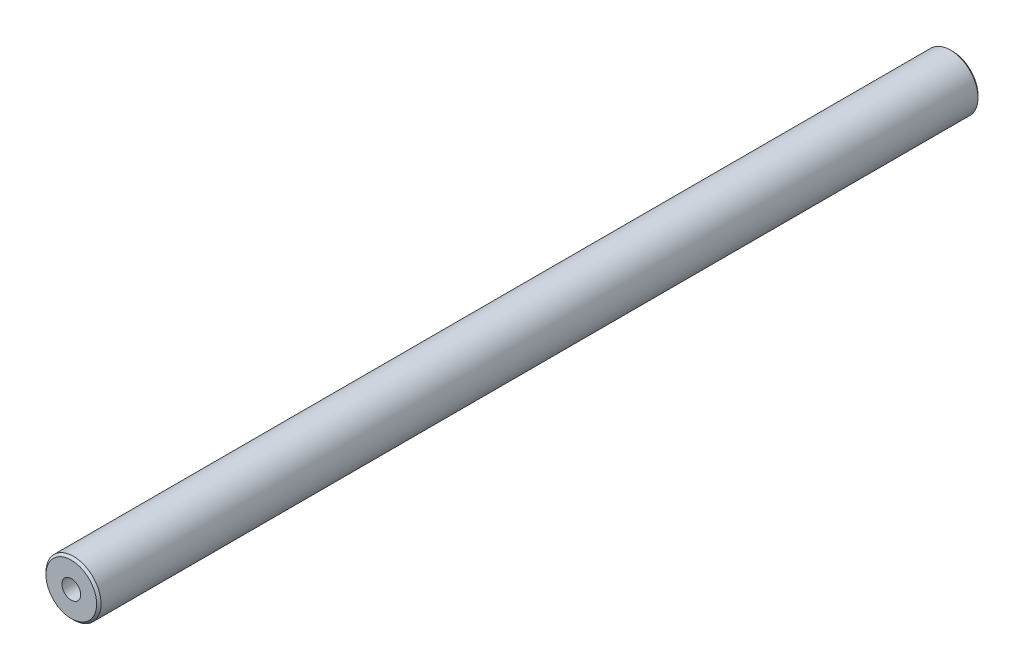
from build123d import *

# Parameters (mm, degrees)
SKETCH_1_R              = 12.5
EXTRUDE_1_DEPTH         = 200
CHAMFER_1_SIZE          = 1
HOLE_WIZARD_M10_1_D     = 8.5
HOLE_WIZARD_M10_1_DEPTH = 24.5
HOLE_WIZARD_M10_1_TIP   = 2.553657631


with BuildPart() as part:
    # 草图1 → 凸台-拉伸1 (new, symmetric)
    with BuildSketch(Plane.XY):
        Circle(SKETCH_1_R)
    extrude(amount=EXTRUDE_1_DEPTH, both=True)

    # 倒角1
    chamfer_1_edges = [part.edges().sort_by_distance(p)[0] for p in [
        (-12.5, 0, -200),
        (-12.5, 0, 200),
    ]]
    chamfer(chamfer_1_edges, length=CHAMFER_1_SIZE)

    # M10 螺纹孔1
    with Locations(Plane.XY.offset(200)):
        with Locations((0, 0)):
            Hole(HOLE_WIZARD_M10_1_D / 2, depth=HOLE_WIZARD_M10_1_DEPTH)
            with Locations((0, 0, -(HOLE_WIZARD_M10_1_DEPTH + HOLE_WIZARD_M10_1_TIP / 2))):  # 118° drill point
                Cone(0, HOLE_WIZARD_M10_1_D / 2, HOLE_WIZARD_M10_1_TIP, mode=Mode.SUBTRACT)


solid = part.part
